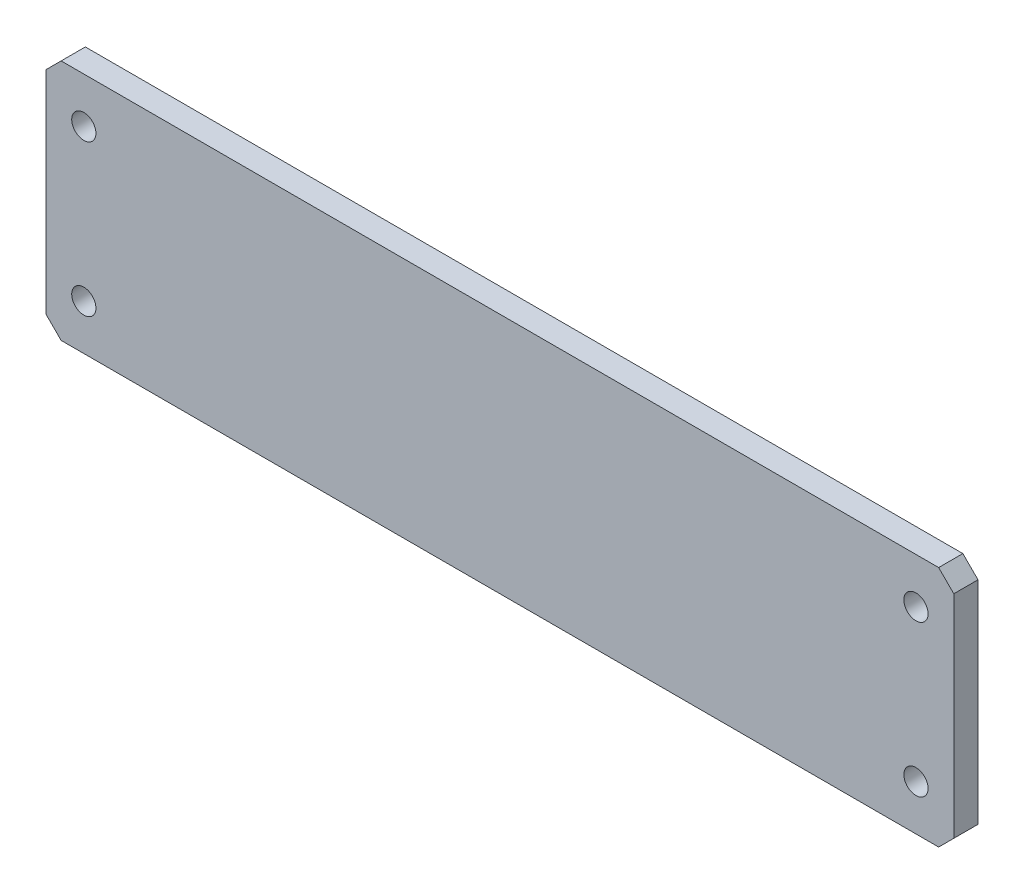
from build123d import *

# Parameters (mm, degrees)
SKETCH1_W           = 300
SKETCH1_H           = 80
BOSS_EXTRUDE1_DEPTH = 8
SKETCH2_R           = 4
CUT_EXTRUDE1_DEPTH  = 8
CHAMFER1_SIZE       = 5


with BuildPart() as part:
    # Sketch1 → Boss-Extrude1 (new body)
    with BuildSketch(Plane.XY):
        Rectangle(SKETCH1_W, SKETCH1_H)
    extrude(amount=BOSS_EXTRUDE1_DEPTH)

    # Sketch2 → Cut-Extrude1 (cut)
    with BuildSketch(Plane.XY.offset(8)):
        with Locations((-137.5, 25)):
            Circle(SKETCH2_R)
        with Locations((-137.5, -25)):
            Circle(SKETCH2_R)
        with Locations((137.5, 25)):
            Circle(SKETCH2_R)
        with Locations((137.5, -25)):
            Circle(SKETCH2_R)
    extrude(amount=-CUT_EXTRUDE1_DEPTH, mode=Mode.SUBTRACT)

    # Chamfer1
    chamfer1_edges = [part.edges().sort_by_distance(p)[0] for p in [
        (-150, -40, 4),
        (-150, 40, 4),
        (150, 40, 4),
        (150, -40, 4),
    ]]
    chamfer(chamfer1_edges, length=CHAMFER1_SIZE)


solid = part.part
